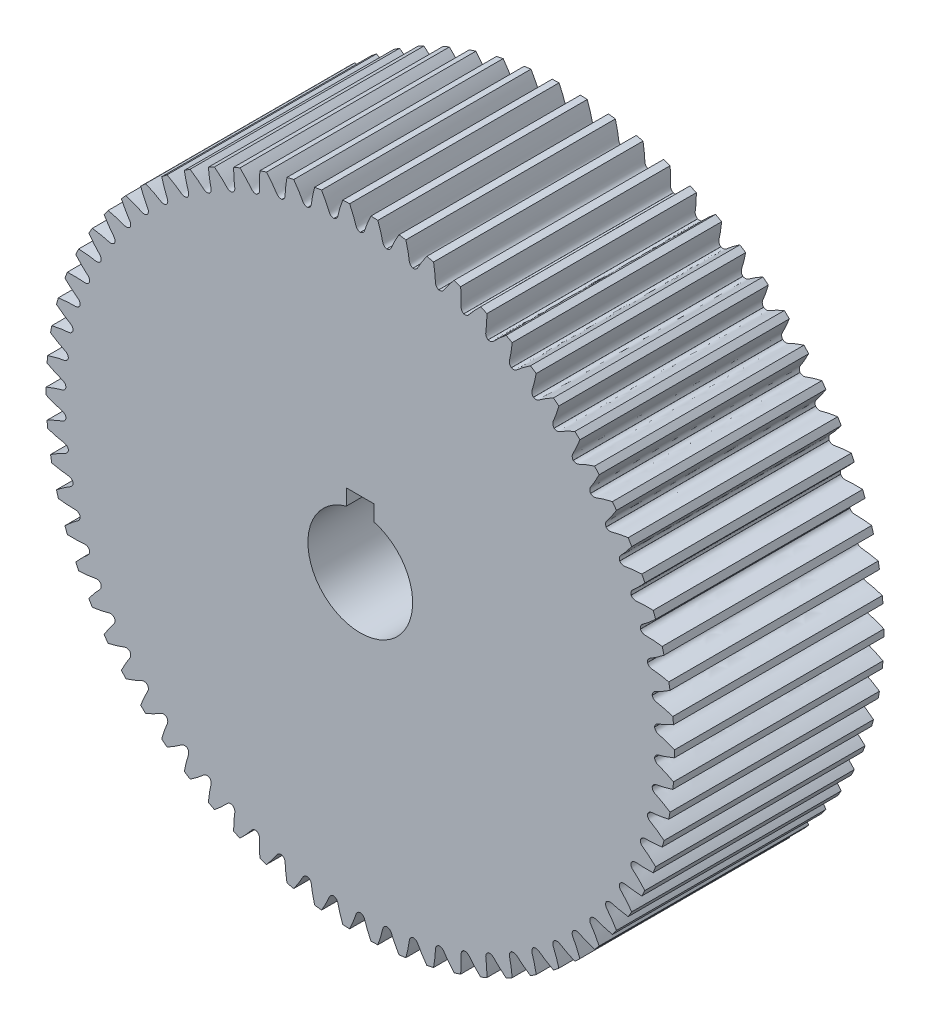
from build123d import *

# Parameters (mm, degrees)
SKETCH_1_R               = 90
EXTRUDE_1_DEPTH          = 60
CUT_EXTRUDE_1_DEPTH      = 141.712472795
PATTERN_CIRCULAR_1_COUNT = 70
SKETCH_4_R               = 15
CUT_EXTRUDE_2_DEPTH      = 141.679472565
SKETCH_5_W               = 8
SKETCH_5_H               = 8
CUT_EXTRUDE_3_DEPTH      = 141.679472565


with BuildPart() as part:
    # 草图1 → 凸台-拉伸1 (new body)
    with BuildSketch(Plane.XY):
        Circle(SKETCH_1_R)
    extrude(amount=EXTRUDE_1_DEPTH)

    # 草图2 → 切除-拉伸1 (cut, through all)
    with BuildSketch(Plane.XY):
        with BuildLine():
            ThreePointArc((0.01, 84.374454327), (0, 84.37445492), (-0.01, 84.374454327))
            add(Edge.make_bspline(
                [(-0.01, 84.374454327), (-1.072397909, 84.588603786), (-1.264388275, 85.530010362), (-1.633622309, 86.591719291), (-1.82385477, 87.118524817), (-2.037524863, 87.671430846), (-2.274330675, 88.250596989), (-2.535815847, 88.855045081), (-2.822961366, 89.484083518), (-3.13688449, 90.136893826), (-3.478635232, 90.812651035), (-3.849253891, 91.510489678), (-4.249753375, 92.229514306), (-4.681123143, 92.968797251), (-5.144326973, 93.727380061), (-5.640302514, 94.504273923), (-6.169960352, 95.29846039), (-6.73418323, 96.108892062), (-7.333825259, 96.934493294), (-7.969711117, 97.774160931), (-8.642635386, 98.626765057), (-9.353361472, 99.491149766), (-10.366637905, 100.67445057), (-11.164425259, 101.55070517), (-11.714959122, 102.132266049)],
                knots=[0, 0, 0, 0, 0.106588038, 0.131121241, 0.157185534, 0.184780915, 0.213907384, 0.244564942, 0.276753589, 0.310473325, 0.345724149, 0.382506062, 0.420819064, 0.460663154, 0.502038333, 0.544944601, 0.589381957, 0.635350402, 0.682849936, 0.731880558, 0.782442269, 0.834535069, 0.888158957, 1, 1, 1, 1], degree=3))
            ThreePointArc((-11.714959122, 102.132266049), (0, 102.801945679), (11.714959122, 102.132266049))
            add(Edge.make_bspline(
                [(0.01, 84.374454327), (1.072397909, 84.588603786), (1.264388275, 85.530010362), (1.633622309, 86.591719291), (1.82385477, 87.118524817), (2.037524863, 87.671430846), (2.274330675, 88.250596989), (2.535815847, 88.855045081), (2.822961366, 89.484083518), (3.13688449, 90.136893826), (3.478635232, 90.812651035), (3.849253891, 91.510489678), (4.249753375, 92.229514306), (4.681123143, 92.968797251), (5.144326973, 93.727380061), (5.640302514, 94.504273923), (6.169960352, 95.29846039), (6.73418323, 96.108892062), (7.333825259, 96.934493294), (7.969711117, 97.774160931), (8.642635386, 98.626765057), (9.353361472, 99.491149766), (10.366637905, 100.67445057), (11.164425259, 101.55070517), (11.714959122, 102.132266049)],
                knots=[0, 0, 0, 0, 0.106588038, 0.131121241, 0.157185534, 0.184780915, 0.213907384, 0.244564942, 0.276753589, 0.310473325, 0.345724149, 0.382506062, 0.420819064, 0.460663154, 0.502038333, 0.544944601, 0.589381957, 0.635350402, 0.682849936, 0.731880558, 0.782442269, 0.834535069, 0.888158957, 1, 1, 1, 1], degree=3))
        make_face()
    cut_extrude_1 = extrude(amount=CUT_EXTRUDE_1_DEPTH, mode=Mode.SUBTRACT)

    # 阵列(圆周)1: 切除-拉伸1 ×70 about axis
    pattern_circular_1_axis = Axis((0, 0, 60), (0, 0, -1))
    for i in range(1, PATTERN_CIRCULAR_1_COUNT):
        add(cut_extrude_1.rotate(pattern_circular_1_axis, i * 360 / PATTERN_CIRCULAR_1_COUNT), mode=Mode.SUBTRACT)

    # 草图4 → 切除-拉伸2 (cut, through all)
    with BuildSketch(Plane.XY.offset(60)):
        Circle(SKETCH_4_R)
    extrude(amount=-CUT_EXTRUDE_2_DEPTH, mode=Mode.SUBTRACT)

    # 草图5 → 切除-拉伸3 (cut, through all)
    with BuildSketch(Plane.XY.offset(60)):
        with Locations((0, 15)):
            Rectangle(SKETCH_5_W, SKETCH_5_H)
    extrude(amount=-CUT_EXTRUDE_3_DEPTH, mode=Mode.SUBTRACT)


solid = part.part
